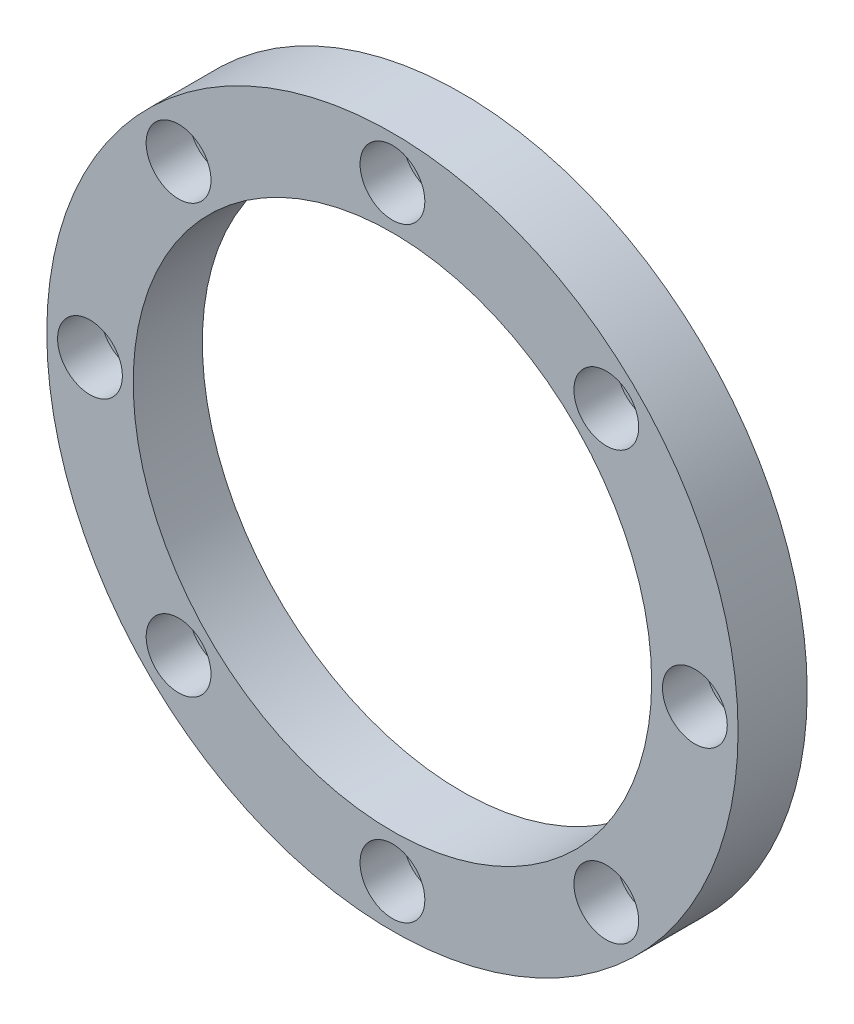
SolidWorks part; units mm, degrees
ref_plane "Front Plane" through (0, 0, 0) normal (0, 0, 1) x (1, 0, 0)
ref_plane "Top Plane" through (0, 0, 0) normal (0, 1, 0) x (1, 0, 0)
ref_plane "Right Plane" through (0, 0, 0) normal (1, 0, 0) x (0, 0, -1)
sketch "Sketch1" plane through (0, 0, 0) normal (0, 0, 1) x (1, 0, 0)
  circle A0 centre (0, 0) radius 40
  circle A1 centre (0, 0) radius 30
  dimension "D1" = 60
  dimension "D2" = 80
extrude "Boss-Extrude1" add sketch "Sketch1" along normal mid plane 8
hole_wizard "Hole Size by Socket Head Cap Screw Type1" positions "Sketch3" profile "Sketch2" counterbore size "M4" standard "Gb" end condition through all
sketch "Sketch3" plane through (0, 0, 4) normal (0, 0, 1) x (1, 0, 0)
  point P4 (35, 0)
  dimension "D1" = 35
sketch "Sketch2" plane through (35, 0, 4) normal (1, 0, 0) x (0, -1, 0)
  line L0 (0, 0) -> (0, 8)
  line L1 (0, 8) -> (2.1, 8)
  line L3 (2.1, 8) -> (2.1, 5)
  line L4 (2.1, 5) -> (3.75, 5)
  line L5 (3.75, 5) -> (3.75, 0)
  line L7 (3.75, 0) -> (0, 0)
  line L11 (0, -6.35) -> (0, 107.95) construction
  dimension "通孔孔直径" = 4.2
  dimension "通孔孔深度" = 8
  dimension "柱形沉头孔直径" = 7.5
  dimension "柱形沉头孔深度" = 5
pattern_circular "CirPattern1" count 8 over 360 about axis through (0, 0, 0) along (0, 0, 1) of "Hole Size by Socket Head Cap Screw Type1"
